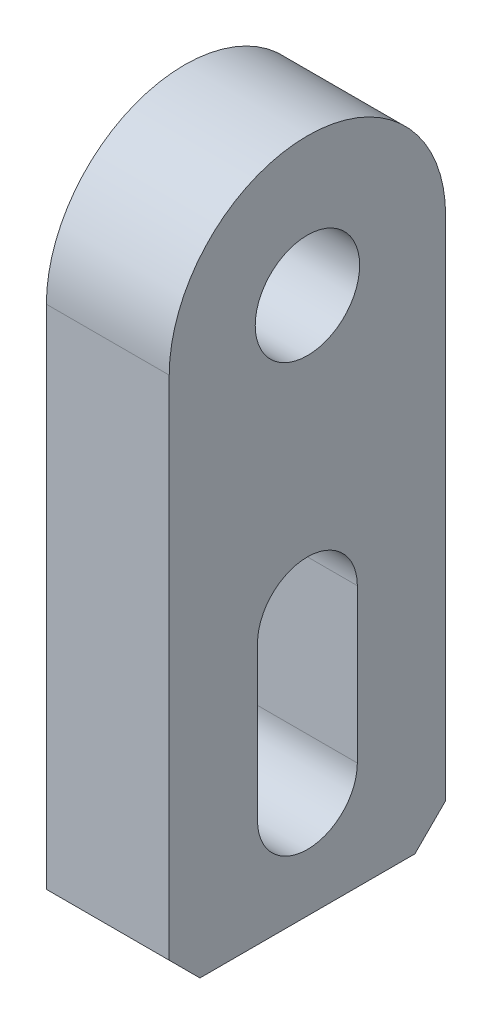
from build123d import *

# Parameters (mm, degrees)
BOSS_EXTRUDE1_DEPTH   = 4
M8_TAPPED_HOLE1_D     = 6.8
M8_TAPPED_HOLE1_DEPTH = 22.25
M8_TAPPED_HOLE1_TIP   = 2.042926105
CHAMFER1_SIZE         = 2


with BuildPart() as part:
    # Sketch1 → Boss-Extrude1 (new, symmetric)
    with BuildSketch(Plane(origin=(0, 0, 0), x_dir=(0, 0, -1), z_dir=(1, 0, 0))):
        with BuildLine():
            Line((-9, 0), (9, 0))
            Line((9, 0), (9, 35))
            ThreePointArc((9, 35), (0, 44), (-9, 35))
            Line((-9, 35), (-9, 0))
        make_face()
        with BuildLine():
            Line((3.25, 17), (3.25, 7))
            ThreePointArc((3.25, 7), (0, 3.75), (-3.25, 7))
            Line((-3.25, 7), (-3.25, 17))
            ThreePointArc((-3.25, 17), (0, 20.25), (3.25, 17))
        make_face(mode=Mode.SUBTRACT)
    extrude(amount=BOSS_EXTRUDE1_DEPTH, both=True)

    # M8 Tapped Hole1
    with Locations(Plane.ZY.offset(4)):
        with Locations((0, 35)):
            Hole(M8_TAPPED_HOLE1_D / 2, depth=M8_TAPPED_HOLE1_DEPTH)
            with Locations((0, 0, -(M8_TAPPED_HOLE1_DEPTH + M8_TAPPED_HOLE1_TIP / 2))):  # 118° drill point
                Cone(0, M8_TAPPED_HOLE1_D / 2, M8_TAPPED_HOLE1_TIP, mode=Mode.SUBTRACT)

    # Chamfer1
    chamfer1_edges = [part.edges().sort_by_distance(p)[0] for p in [
        (0, 0, -9),
        (0, 0, 9),
    ]]
    chamfer(chamfer1_edges, length=CHAMFER1_SIZE)


solid = part.part
